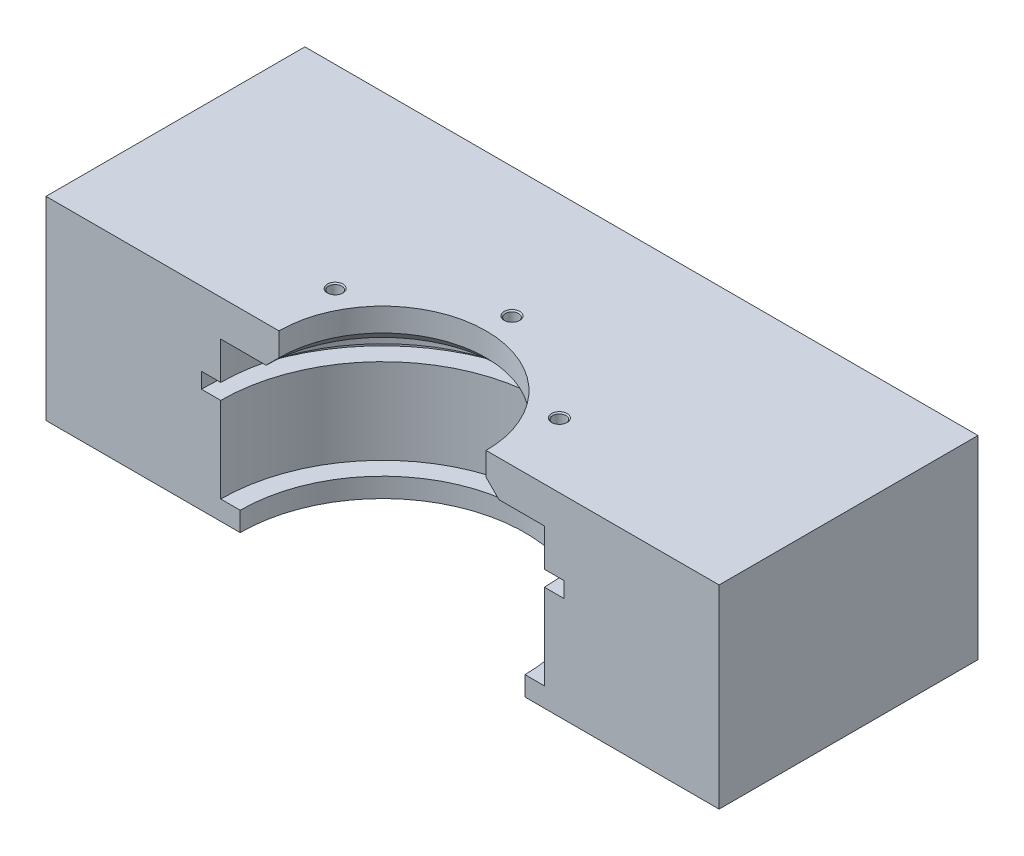
SolidWorks part; units mm, degrees
ref_plane "前视基准面" through (0, 0, 0) normal (0, 0, 1) x (1, 0, 0)
ref_plane "上视基准面" through (0, 0, 0) normal (0, 1, 0) x (1, 0, 0)
ref_plane "右视基准面" through (0, 0, 0) normal (1, 0, 0) x (0, 0, -1)
sketch "草图1" plane through (0, 0, 0) normal (0, 1, 0) x (1, 0, 0)
  line L1 (0, 0) -> (-520, 0)
  line L2 (0, 0) -> (0, 200)
  line L3 (0, 200) -> (-520, 200)
  line L4 (-520, 0) -> (-520, 200)
  dimension "D1" = 200
  dimension "D2" = 520
extrude "凸台-拉伸1" add sketch "草图1" along normal blind 150
sketch "草图2" plane through (0, 150, 0) normal (0, 1, 0) x (1, 0, 0)
  line L0 (-260, 256.6795) -> (-260, -79.7206) construction
  line L1 (0, 0) -> (0, 200) construction
  dimension "D1" = 260
hole_wizard "M12 螺纹孔1" positions "草图3" profile "草图4" tap size "M12" standard "GB"
sketch "草图3" plane through (0, 150, 0) normal (0, 1, 0) x (1, 0, 0)
  line L0 (-260, 256.6795) -> (-260, -79.7206) construction
  line L1 (-520, 0) -> (0, 0) construction
  line L2 (-260, 0) -> (-173.3975, 50) construction
  line L4 (-260, 0) -> (-260, 100) construction
  circle A0 centre (-260, 0) radius 100 construction
  point P0 (-260, 100)
  point P11 (-173.3975, 50)
  point P25 (-346.6025, 50)
  dimension "D1" = 200
  dimension "D2" = 30
sketch "草图4" plane through (-260, 150, -100) normal (1, 0, 0) x (0, 0, 1)
  line L0 (0, 0) -> (0, 18.0644)
  line L1 (0, 18.0644) -> (5.1, 15)
  line L2 (5.1, 15) -> (5.1, 0.925)
  line L3 (5.1, 0.925) -> (6.025, 0)
  line L5 (6.025, 0) -> (0, 0)
  line L6 (-5.1, 0.925) -> (-6.025, 0) construction
  line L10 (0, 18.0644) -> (-5.1, 15) construction
  line L11 (0, -6.35) -> (0, 107.95) construction
  dimension "螺纹孔钻头直径" = 10.2
  dimension "螺纹孔钻头深度" = 15
  dimension "近端锥形沉头孔直径" = 12.05
  dimension "近端锥形沉头孔角度" = 90
  dimension "导头角度" = 118
cosmetic thread "孔螺蚊线1" parameters "D1"=17, "D2"=12
cosmetic thread "孔螺蚊线2" parameters "D1"=17, "D2"=12
cosmetic thread "孔螺蚊线3" parameters "D1"=17, "D2"=12
sketch "草图6" plane through (0, 0, 0) normal (0, 0, 1) x (1, 0, 0)
  line L0 (-260, 150) -> (-340, 150)
  line L1 (-520, 150) -> (0, 150) construction
  line L2 (-340, 150) -> (-340, 122)
  line L3 (-340, 122) -> (-385, 122)
  line L4 (-385, 122) -> (-385, 93)
  line L5 (-385, 93) -> (-400, 93)
  line L6 (-400, 93) -> (-400, 81)
  line L7 (-400, 81) -> (-385, 81)
  line L8 (-385, 81) -> (-385, 15)
  line L9 (-385, 15) -> (-370, 15)
  line L10 (-370, 15) -> (-370, 0)
  line L11 (-520, 0) -> (0, 0) construction
  line L12 (-370, 0) -> (-260, 0)
  line L13 (-260, 0) -> (-260, 150)
  point P4 (-377.5, 15)
  dimension "D1" = 80
  dimension "D2" = 125
  dimension "D3" = 110
  dimension "D4" = 125
  dimension "D5" = 140
  dimension "D6" = 12
  dimension "D7" = 107
  dimension "D8" = 135
  dimension "D9" = 78
revolve "切除-旋转1" cut sketch "草图6" angle 360 about L13
chamfer "倒角1" distance 10 angle 45 1 edges at (-260, 122, -80)
